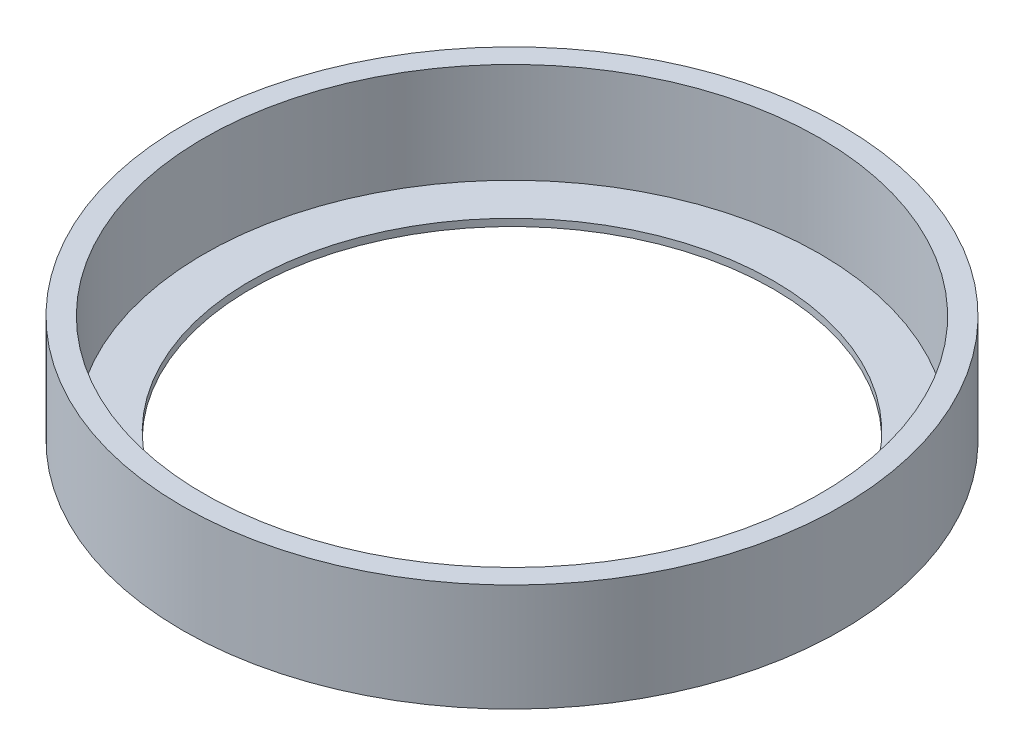
SolidWorks part; units mm, degrees
ref_plane "前视基准面" through (0, 0, 0) normal (0, 0, 1) x (1, 0, 0)
ref_plane "上视基准面" through (0, 0, 0) normal (0, 1, 0) x (1, 0, 0)
ref_plane "右视基准面" through (0, 0, 0) normal (1, 0, 0) x (0, 0, -1)
sketch "草图1" plane through (0, 0, 0) normal (0, 0, 1) x (1, 0, 0)
  line L0 (-46, 15) -> (-46, 0)
  line L1 (-46, 0) -> (-36.5, 0)
  line L2 (-36.5, 0) -> (-36.5, 1)
  line L3 (-36.5, 1) -> (-43, 1)
  line L4 (-43, 1) -> (-43, 15)
  line L5 (-43, 15) -> (-46, 15)
  line L6 (0, 0) -> (0, 8.1892) construction
  point P9 (-36.5, 0.5)
  dimension "D1" = 1
  dimension "D2" = 73
  dimension "D3" = 86
  dimension "D4" = 92
  dimension "D5" = 15
revolve "旋转1" add sketch "草图1" angle 360 about L6
equation "\"图号代码1\"= \"图号代码\""
equation "\"名称代码2\"= \"名称代码\""
